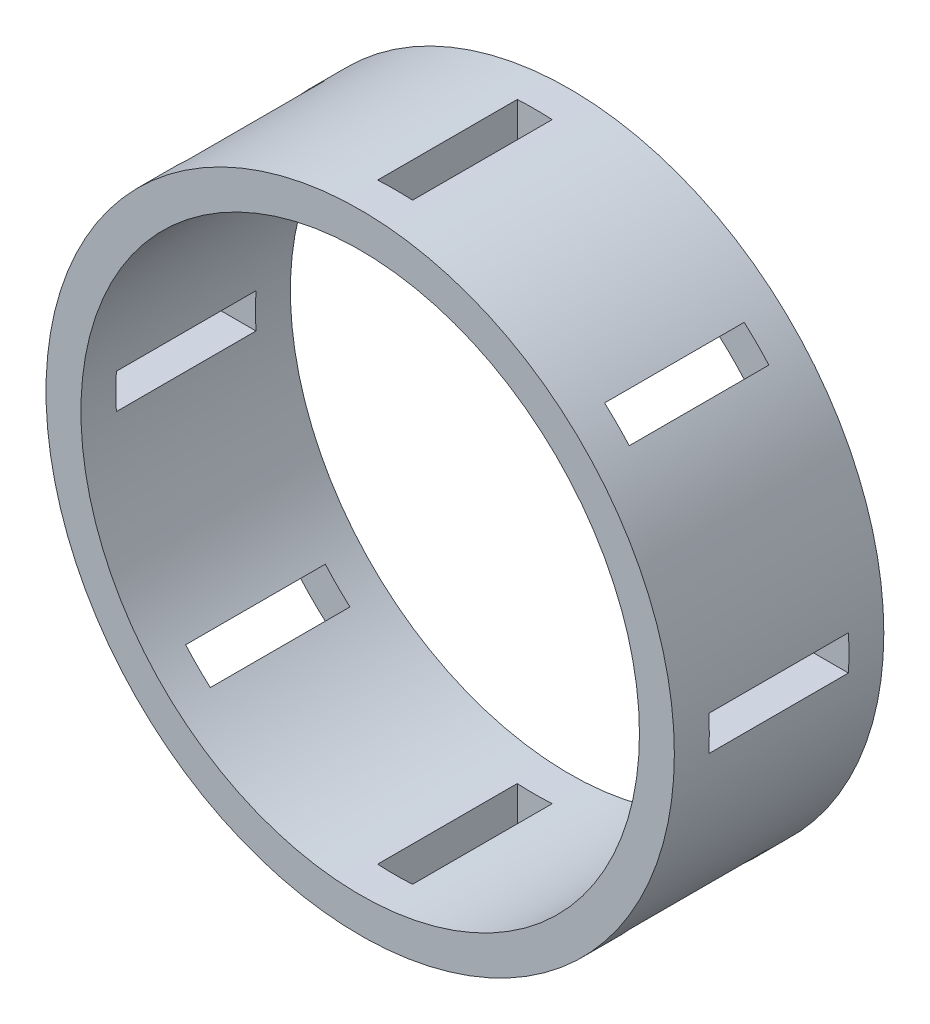
from build123d import *

# Parameters (mm, degrees)
SKETCH1_R           = 45
SKETCH1_R_2         = 40
BOSS_EXTRUDE1_DEPTH = 30
SKETCH2_W           = 5
SKETCH2_H           = 20
CUT_EXTRUDE1_DEPTH  = 660.545773414
CIRPATTERN1_COUNT   = 8


with BuildPart() as part:
    # Sketch1 → Boss-Extrude1 (new body)
    with BuildSketch(Plane.XY):
        with Locations((-599.884196758, -90)):
            Circle(SKETCH1_R)
        with Locations((-599.884196758, -90)):
            Circle(SKETCH1_R_2, mode=Mode.SUBTRACT)
    extrude(amount=BOSS_EXTRUDE1_DEPTH)

    # Sketch2 → Cut-Extrude1 (cut, symmetric)
    with BuildSketch(Plane(origin=(0, 0, 0), x_dir=(1, 0, 0), z_dir=(0, 1, 0))):
        with Locations((-599.884196758, -15)):
            Rectangle(SKETCH2_W, SKETCH2_H)
    cut_extrude1 = extrude(amount=CUT_EXTRUDE1_DEPTH, both=True, mode=Mode.SUBTRACT)

    # CirPattern1: Cut-Extrude1 ×8 about axis
    cirpattern1_axis = Axis((-599.884196758, -90, 0), (0, 0, 1))
    for i in range(1, CIRPATTERN1_COUNT):
        add(cut_extrude1.rotate(cirpattern1_axis, i * 360 / CIRPATTERN1_COUNT), mode=Mode.SUBTRACT)


solid = part.part
